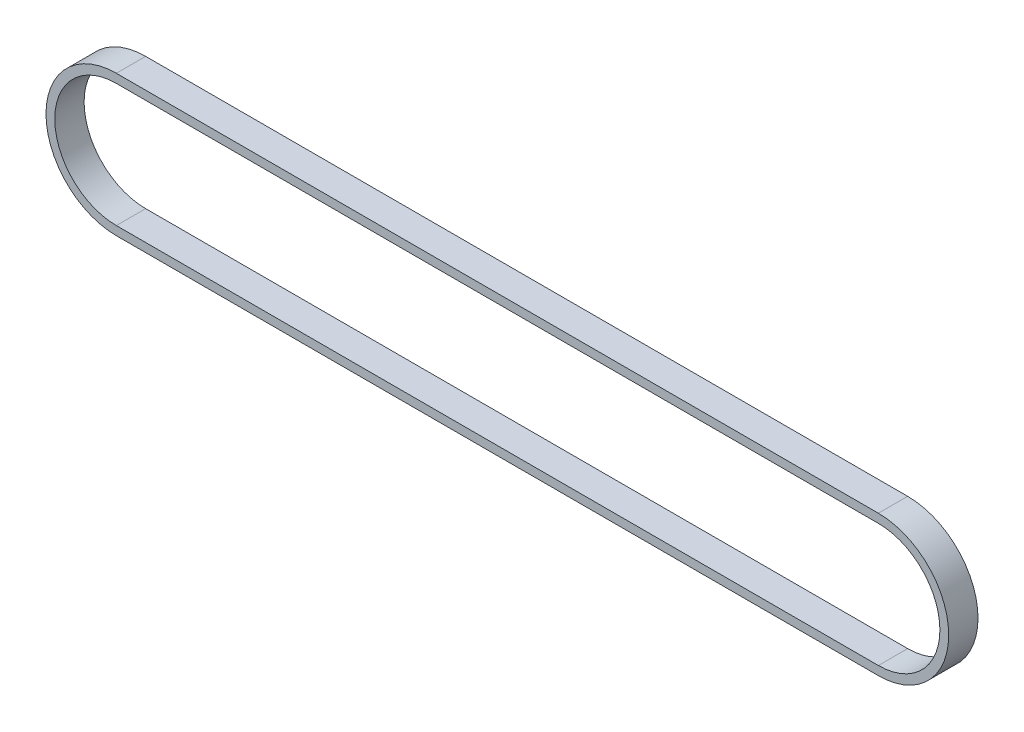
SolidWorks part; units mm, degrees
ref_plane "Front Plane" through (0, 0, 0) normal (0, 0, 1) x (1, 0, 0)
ref_plane "Top Plane" through (0, 0, 0) normal (0, 1, 0) x (1, 0, 0)
ref_plane "Right Plane" through (0, 0, 0) normal (1, 0, 0) x (0, 0, -1)
sketch "Sketch2" plane through (0, 0, 0) normal (0, 0, 1) x (1, 0, 0)
  line L0 (5.5, 0) -> (-5.5, 0) construction
  line L1 (0, 24) -> (-260, 24)
  line L2 (0, -24) -> (-260, -24)
  arc A0 (0, -24) -> (0, 24) centre (0, 0) ccw
  arc A1 (-260, 24) -> (-260, -24) centre (-260, 0) ccw
  dimension "D1" = 48
  dimension "D2" = 48
  dimension "D3" = 260
extrude "Boss-Extrude1" add sketch "Sketch2" along normal blind 10
shell "Shell1" thickness 3
